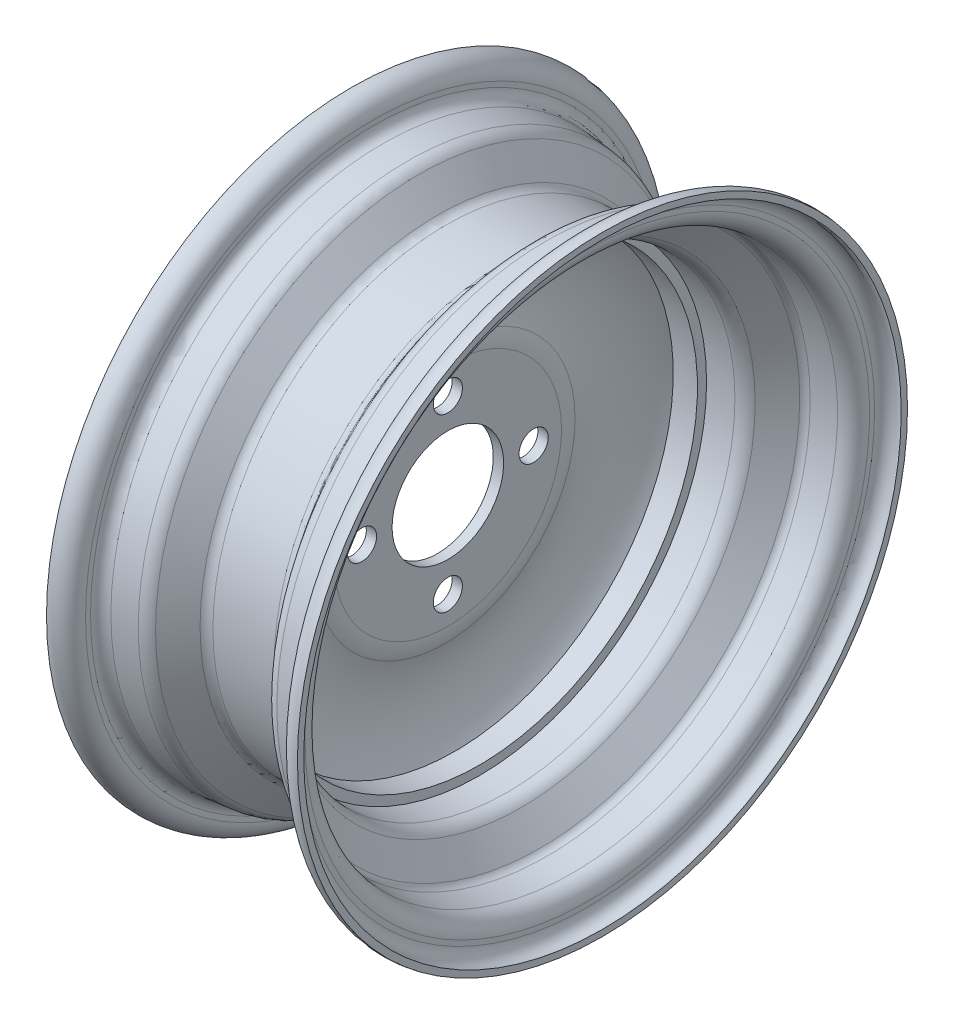
SolidWorks part; units mm, degrees
material "7079 合金"
ref_plane "前视基准面" through (0, 0, 0) normal (0, 0, 1) x (1, 0, 0)
ref_plane "上视基准面" through (0, 0, 0) normal (0, 1, 0) x (1, 0, 0)
ref_plane "右视基准面" through (0, 0, 0) normal (1, 0, 0) x (0, 0, -1)
sketch "草图1" plane through (0, 0, 0) normal (0, 0, 1) x (1, 0, 0)
  line L23 (84.4803, 317.7627) -> (83.8413, 320.3941)
  line L26 (96.4554, 268.4534) -> (84.4803, 317.7627)
  line L27 (97.0221, 268.0882) -> (96.9199, 268.0882)
  line L28 (97.5, 244.8015) -> (97.5, 267.6103)
  line L29 (96.8899, 244.3235) -> (97.0221, 244.3235)
  line L30 (78.5236, 193.1098) -> (96.4391, 244.0043)
  line L31 (79.1815, 192.6755) -> (78.6405, 192.866)
  line L32 (79.1079, 191.8907) -> (79.2983, 192.4317)
  line L33 (78.3231, 191.9643) -> (78.8641, 191.7739)
  line L34 (77.0954, 189.0523) -> (78.0793, 191.8475)
  line L35 (77.7532, 188.6181) -> (77.2122, 188.8085)
  line L36 (77.6796, 187.8333) -> (77.8701, 188.3743)
  line L37 (76.8948, 187.9069) -> (77.4358, 187.7165)
  line L38 (75.6671, 184.9949) -> (76.651, 187.79)
  line L39 (76.325, 184.5607) -> (75.784, 184.7511)
  line L40 (76.2514, 183.7759) -> (76.4418, 184.3169)
  line L41 (75.4666, 183.8495) -> (76.0076, 183.659)
  line L42 (73.1324, 177.7941) -> (75.2228, 183.7326)
  line L43 (59.75, 177.7941) -> (73.1324, 177.7941)
  line L44 (59.75, 162.5) -> (59.75, 177.7941)
  line L45 (50.25, 162.5) -> (59.75, 162.5)
  line L46 (50.25, 187.3529) -> (50.25, 162.5)
  line L47 (66.4222, 187.3529) -> (50.25, 187.3529)
  line L48 (88.0074, 248.6723) -> (66.4222, 187.3529)
  line L49 (88.0074, 263.1405) -> (88.0074, 248.6723)
  line L50 (75.7794, 313.4968) -> (88.0074, 263.1405)
  line L51 (-66.4905, 320.8) -> (66.4905, 320.8)
  line L52 (-88.0074, 263.1405) -> (-75.7794, 313.4968)
  line L53 (-88.0074, 248.6723) -> (-88.0074, 263.1405)
  line L54 (-66.4222, 187.3529) -> (-88.0074, 248.6723)
  line L55 (-50.25, 187.3529) -> (-66.4222, 187.3529)
  line L56 (-50.25, 162.5) -> (-50.25, 187.3529)
  line L57 (-59.75, 162.5) -> (-50.25, 162.5)
  line L58 (-59.75, 177.7941) -> (-59.75, 162.5)
  line L59 (-73.1324, 177.7941) -> (-59.75, 177.7941)
  line L60 (-75.2228, 183.7326) -> (-73.1324, 177.7941)
  line L61 (-76.0076, 183.659) -> (-75.4666, 183.8495)
  line L62 (-76.4418, 184.3169) -> (-76.2514, 183.7759)
  line L63 (-75.784, 184.7511) -> (-76.325, 184.5607)
  line L64 (-76.651, 187.79) -> (-75.6671, 184.9949)
  line L65 (-77.4358, 187.7165) -> (-76.8948, 187.9069)
  line L66 (-77.8701, 188.3743) -> (-77.6796, 187.8333)
  line L67 (-77.2122, 188.8085) -> (-77.7532, 188.6181)
  line L68 (-78.0793, 191.8475) -> (-77.0954, 189.0523)
  line L69 (-78.8641, 191.7739) -> (-78.3231, 191.9643)
  line L70 (-79.2983, 192.4317) -> (-79.1079, 191.8907)
  line L71 (-78.6405, 192.866) -> (-79.1815, 192.6755)
  line L72 (-96.4391, 244.0043) -> (-78.5236, 193.1098)
  line L73 (-97.0221, 244.3235) -> (-96.8899, 244.3235)
  line L74 (-97.5, 267.6103) -> (-97.5, 244.8015)
  line L75 (-96.9199, 268.0882) -> (-97.0221, 268.0882)
  line L76 (-83.8413, 320.3941) -> (-96.4554, 268.4534)
  line L80 (0, 0) -> (0, 335) construction
  line L81 (-50.25, 162.5) -> (50.25, 162.5) construction
  line L82 (0, 0) -> (328.2798, 0) construction
  line L83 (-65.2636, 335) -> (65.2636, 335)
  arc A1 (-65.2636, 335) -> (-83.8413, 320.3941) centre (-65.2636, 315.8824) ccw
  arc A2 (83.8413, 320.3941) -> (65.2636, 335) centre (65.2636, 315.8824) ccw
  arc A10 (96.4554, 268.4534) -> (96.9199, 268.0882) centre (96.9199, 268.5662) ccw
  arc A11 (97.5, 267.6103) -> (97.0221, 268.0882) centre (97.0221, 267.6103) ccw
  arc A12 (97.0221, 244.3235) -> (97.5, 244.8015) centre (97.0221, 244.8015) ccw
  arc A13 (96.8899, 244.3235) -> (96.4391, 244.0043) centre (96.8899, 243.8456) ccw
  arc A14 (78.5236, 193.1098) -> (78.6405, 192.866) centre (78.704, 193.0463) ccw
  arc A15 (79.2983, 192.4317) -> (79.1815, 192.6755) centre (79.118, 192.4952) ccw
  arc A16 (78.8641, 191.7739) -> (79.1079, 191.8907) centre (78.9276, 191.9542) ccw
  arc A17 (78.3231, 191.9643) -> (78.0793, 191.8475) centre (78.2596, 191.784) ccw
  arc A18 (77.0954, 189.0523) -> (77.2122, 188.8085) centre (77.2757, 188.9889) ccw
  arc A19 (77.8701, 188.3743) -> (77.7532, 188.6181) centre (77.6897, 188.4378) ccw
  arc A20 (77.4358, 187.7165) -> (77.6796, 187.8333) centre (77.4993, 187.8968) ccw
  arc A21 (76.8948, 187.9069) -> (76.651, 187.79) centre (76.8314, 187.7266) ccw
  arc A22 (75.6671, 184.9949) -> (75.784, 184.7511) centre (75.8474, 184.9314) ccw
  arc A23 (76.4418, 184.3169) -> (76.325, 184.5607) centre (76.2615, 184.3803) ccw
  arc A24 (76.0076, 183.659) -> (76.2514, 183.7759) centre (76.071, 183.8394) ccw
  arc A25 (75.4666, 183.8495) -> (75.2228, 183.7326) centre (75.4031, 183.6691) ccw
  arc A26 (75.7794, 313.4968) -> (66.4905, 320.8) centre (66.4905, 311.2412) ccw
  arc A27 (-66.4905, 320.8) -> (-75.7794, 313.4968) centre (-66.4905, 311.2412) ccw
  arc A28 (-75.2228, 183.7326) -> (-75.4666, 183.8495) centre (-75.4031, 183.6691) ccw
  arc A29 (-76.2514, 183.7759) -> (-76.0076, 183.659) centre (-76.071, 183.8394) ccw
  arc A30 (-76.325, 184.5607) -> (-76.4418, 184.3169) centre (-76.2615, 184.3803) ccw
  arc A31 (-75.784, 184.7511) -> (-75.6671, 184.9949) centre (-75.8474, 184.9314) ccw
  arc A32 (-76.651, 187.79) -> (-76.8948, 187.9069) centre (-76.8314, 187.7266) ccw
  arc A33 (-77.6796, 187.8333) -> (-77.4358, 187.7165) centre (-77.4993, 187.8968) ccw
  arc A34 (-77.7532, 188.6181) -> (-77.8701, 188.3743) centre (-77.6897, 188.4378) ccw
  arc A35 (-77.2122, 188.8085) -> (-77.0954, 189.0523) centre (-77.2757, 188.9889) ccw
  arc A36 (-78.0793, 191.8475) -> (-78.3231, 191.9643) centre (-78.2596, 191.784) ccw
  arc A37 (-79.1079, 191.8907) -> (-78.8641, 191.7739) centre (-78.9276, 191.9542) ccw
  arc A38 (-79.1815, 192.6755) -> (-79.2983, 192.4317) centre (-79.118, 192.4952) ccw
  arc A39 (-78.6405, 192.866) -> (-78.5236, 193.1098) centre (-78.704, 193.0463) ccw
  arc A40 (-96.4391, 244.0043) -> (-96.8899, 244.3235) centre (-96.8899, 243.8456) ccw
  arc A41 (-97.5, 244.8015) -> (-97.0221, 244.3235) centre (-97.0221, 244.8015) ccw
  arc A42 (-97.0221, 268.0882) -> (-97.5, 267.6103) centre (-97.0221, 267.6103) ccw
  arc A43 (-96.9199, 268.0882) -> (-96.4554, 268.4534) centre (-96.9199, 268.5662) ccw
  dimension "D2" = 14.2
  dimension "D3" = 0.4779
  dimension "D4" = 0.1912
  dimension "D5" = 9.5588
  dimension "D1" = 670
  dimension "D6" = 325
  dimension "D7" = 195
  dimension "D8" = 119.5
  dimension "D9" = 9.5
  dimension "D10" = 24.8529
  dimension "D11" = 15.2941
  dimension "D12" = 146.2647
sketch "草图2" plane through (0, 0, 0) normal (0, 0, 1) x (1, 0, 0)
  line L0 (55.0334, 158.3536) -> (40.3872, 157.0722)
  line L1 (60.7057, 167.4531) -> (60.7057, 164.5438)
  line L2 (73.1324, 174.1159) -> (73.1324, 177.7941)
  line L3 (64.2904, 164.5438) -> (64.2904, 167.4531)
  line L4 (40.6996, 153.5011) -> (55.3459, 154.7825)
  line L5 (25.683, 136.4516) -> (36.7734, 151.3128)
  line L6 (1.3, 132.5134) -> (17.8301, 132.5134)
  line L7 (1.3, 127.1981) -> (1.3, 132.5134)
  line L8 (-12.8027, 127.1981) -> (1.3, 127.1981)
  line L9 (-17, 32.5) -> (-17, 66.2738)
  line L10 (-23, 32.5) -> (-17, 32.5)
  line L11 (-23, 68.6619) -> (-23, 32.5)
  line L12 (-36.7734, 151.3128) -> (-25.683, 136.4516)
  line L13 (-55.3459, 154.7825) -> (-40.6996, 153.5011)
  line L14 (-64.2904, 167.4531) -> (-64.2904, 164.5438)
  line L15 (-73.1324, 177.7941) -> (-73.1324, 174.1159)
  line L16 (-60.7057, 164.5438) -> (-60.7057, 167.4531)
  line L17 (-40.3872, 157.0722) -> (-55.0334, 158.3536)
  line L18 (-22.8101, 138.5956) -> (-33.9004, 153.4568)
  line L19 (17.8301, 136.0981) -> (-17.8301, 136.0981)
  line L20 (33.9004, 153.4568) -> (22.8101, 138.5956)
  line L21 (-73.1324, 175.955) -> (73.1324, 175.955) construction
  line L22 (0, 175.955) -> (0, 175.971) construction
  line L23 (0, 0) -> (328.2798, 0) construction
  line L24 (0, 0) -> (0, 335) construction
  line L25 (0, 0) -> (328.2798, 0) construction
  line L26 (0, 0) -> (0, 335) construction
  line L28 (-26.6192, 55.5) -> (-19.2091, 55.5) construction
  line L29 (-26.6192, 55.5) -> (-26.6192, 44.5) construction
  line L30 (-26.6192, 44.5) -> (-19.2091, 44.5) construction
  line L31 (-19.2091, 55.5) -> (-19.2091, 44.5) construction
  arc A0 (40.3872, 157.0722) -> (33.9004, 153.4568) centre (41.1787, 148.0253) ccw
  arc A1 (55.0334, 158.3536) -> (60.7057, 164.5438) centre (54.4919, 164.5438) ccw
  arc A2 (73.1324, 177.7941) -> (60.7057, 167.4531) centre (71.2218, 167.4531) ccw
  arc A3 (73.1324, 174.1159) -> (64.2904, 167.4531) centre (71.2218, 167.4531) ccw
  arc A4 (55.3459, 154.7825) -> (64.2904, 164.5438) centre (54.4919, 164.5438) ccw
  arc A5 (40.6996, 153.5011) -> (36.7734, 151.3128) centre (41.1787, 148.0253) ccw
  arc A6 (17.8301, 132.5134) -> (25.683, 136.4516) centre (17.8301, 142.3119) ccw
  arc A10 (-23, 68.6619) -> (-24.0652, 75.6614) centre (-46.5292, 68.6619) ccw
  arc A13 (-25.683, 136.4516) -> (-12.8027, 133.9014) centre (-17.8301, 142.3119) ccw
  arc A14 (-36.7734, 151.3128) -> (-40.6996, 153.5011) centre (-41.1787, 148.0253) ccw
  arc A15 (-64.2904, 164.5438) -> (-55.3459, 154.7825) centre (-54.4919, 164.5438) ccw
  arc A16 (-64.2904, 167.4531) -> (-73.1324, 174.1159) centre (-71.2218, 167.4531) ccw
  arc A17 (-60.7057, 167.4531) -> (-73.1324, 177.7941) centre (-71.2218, 167.4531) ccw
  arc A18 (-60.7057, 164.5438) -> (-55.0334, 158.3536) centre (-54.4919, 164.5438) ccw
  arc A19 (-33.9004, 153.4568) -> (-40.3872, 157.0722) centre (-41.1787, 148.0253) ccw
  arc A20 (-22.8101, 138.5956) -> (-17.8301, 136.0981) centre (-17.8301, 142.3119) ccw
  arc A21 (17.8301, 136.0981) -> (22.8101, 138.5956) centre (17.8301, 142.3119) ccw
  arc A24 (-12.8027, 133.9014) -> (-24.0652, 75.6614) centre (35.7581, 94.3017) ccw
  arc A25 (-12.8027, 127.1981) -> (-18.5066, 75.6614) centre (40.7561, 95.1864) ccw
  arc A26 (-17, 66.2738) -> (-18.5066, 75.6614) centre (-47, 66.2738) ccw
  point P0 (-0.029, 0.0006)
  point P19 (-19.2091, 50)
  dimension "D3" = 9.0815
  dimension "D4" = 6
  dimension "D5" = 8.9
  dimension "D6" = 2.6
  dimension "D7" = 11
  dimension "D8" = 34
  dimension "D9" = 100
  dimension "D1" = 30
  dimension "D2" = 65
revolve "旋转1" add sketch "草图2" angle 360 about L82
sketch "草图3" plane through (-23, 0, 0) normal (-1, 0, 0) x (0, 0, 1)
  line L0 (0, 0) -> (0, 335) construction
  circle A0 centre (0, 50) radius 8.5
  circle A1 centre (0, 0) radius 50 construction
  circle A2 centre (50, 0) radius 8.5
  circle A3 centre (0, -50) radius 8.5
  circle A4 centre (-50, 0) radius 8.5
  point P18 (0, 0)
  dimension "D1" = 100
  dimension "D2" = 17
  dimension "D3" = 4
extrude "切除-拉伸1" cut sketch "草图3" against normal through all
